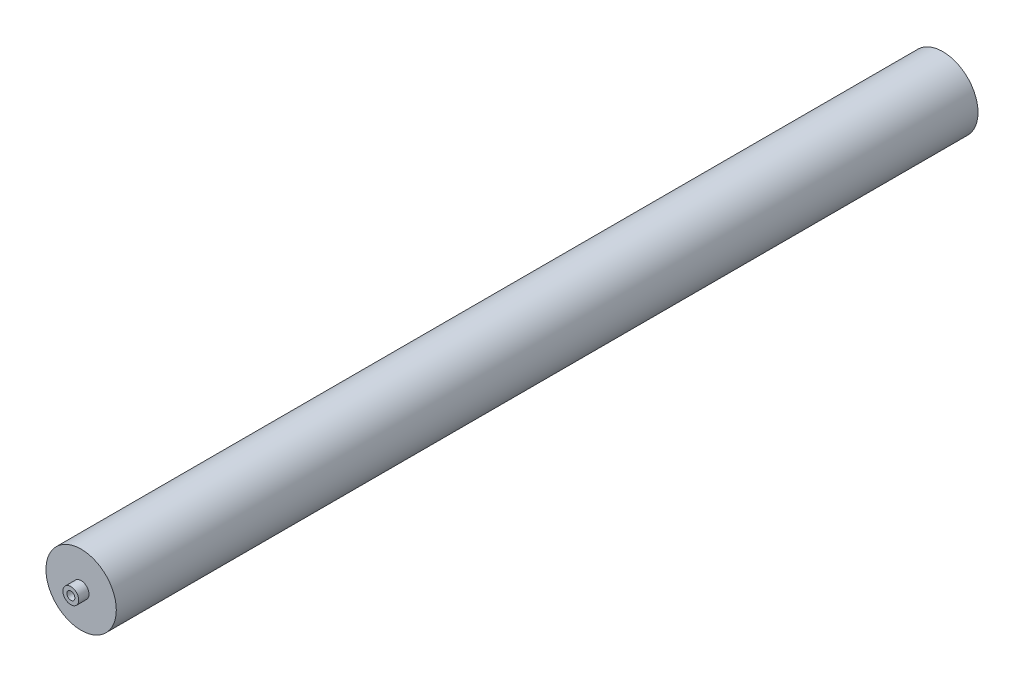
from build123d import *

# Parameters (mm, degrees)
SKETCH1_R              = 44.5
BOSS_EXTRUDE1_DEPTH    = 1090
SKETCH2_R              = 10
BOSS_EXTRUDE2_DEPTH    = 13
BOSS_EXTRUDE3_START    = 13
SKETCH3_R              = 10
BOSS_EXTRUDE3_DEPTH    = 13
M12_TAPPED_HOLE1_D     = 10.2
M12_TAPPED_HOLE1_DEPTH = 25.25
M12_TAPPED_HOLE1_TIP   = 3.064389157
M12_TAPPED_HOLE2_D     = 10.2
M12_TAPPED_HOLE2_DEPTH = 25.25
M12_TAPPED_HOLE2_TIP   = 3.064389157


with BuildPart() as part:
    # Sketch1 → Boss-Extrude1 (new body)
    with BuildSketch(Plane.XY):
        Circle(SKETCH1_R)
    extrude(amount=BOSS_EXTRUDE1_DEPTH)

    # Sketch2 → Boss-Extrude2 (add)
    with BuildSketch(Plane.XY.offset(1090)):
        with Locations(Location((0, 0, 0), (0, 0, 180))):
            Circle(SKETCH2_R)
    extrude(amount=BOSS_EXTRUDE2_DEPTH)

    # Sketch3 → Boss-Extrude3 (add)
    with BuildSketch(Plane(origin=(0, 0, 0), x_dir=(-1, 0, 0), z_dir=(0, 0, -1)).offset(BOSS_EXTRUDE3_START)):
        Circle(SKETCH3_R)
    extrude(amount=-BOSS_EXTRUDE3_DEPTH)

    # M12 Tapped Hole1
    with Locations(Plane(origin=(0, 0, -13), x_dir=(-1, 0, 0), z_dir=(0, 0, -1))):
        with Locations((0, 0)):
            Hole(M12_TAPPED_HOLE1_D / 2, depth=M12_TAPPED_HOLE1_DEPTH)
            with Locations((0, 0, -(M12_TAPPED_HOLE1_DEPTH + M12_TAPPED_HOLE1_TIP / 2))):  # 118° drill point
                Cone(0, M12_TAPPED_HOLE1_D / 2, M12_TAPPED_HOLE1_TIP, mode=Mode.SUBTRACT)

    # M12 Tapped Hole2
    with Locations(Plane.XY.offset(1103)):
        with Locations((0, 0)):
            Hole(M12_TAPPED_HOLE2_D / 2, depth=M12_TAPPED_HOLE2_DEPTH)
            with Locations((0, 0, -(M12_TAPPED_HOLE2_DEPTH + M12_TAPPED_HOLE2_TIP / 2))):  # 118° drill point
                Cone(0, M12_TAPPED_HOLE2_D / 2, M12_TAPPED_HOLE2_TIP, mode=Mode.SUBTRACT)


solid = part.part
